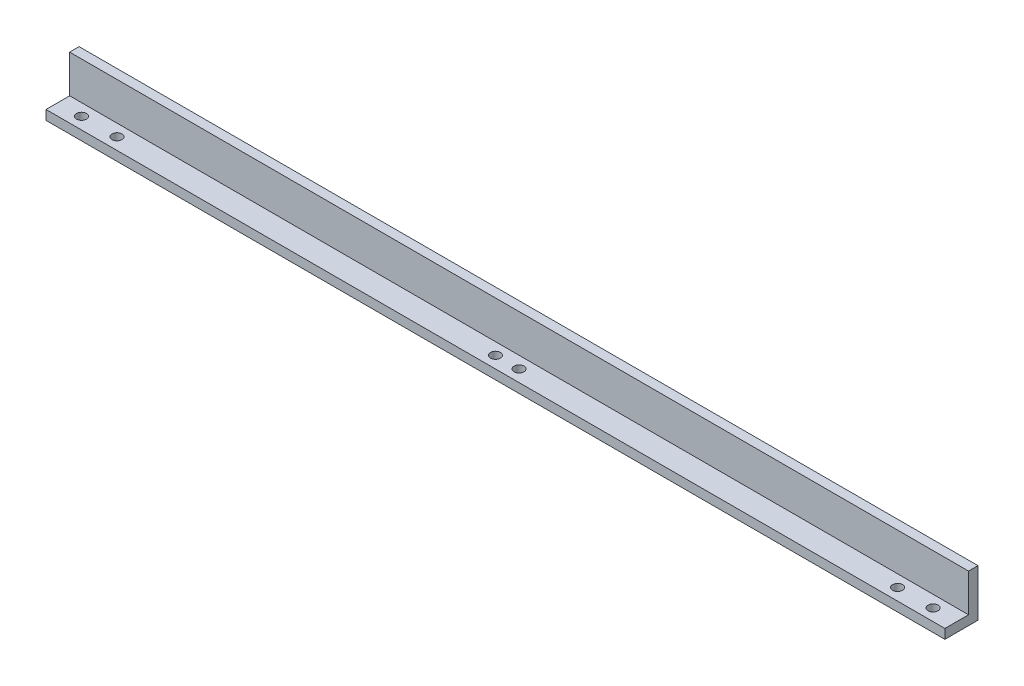
SolidWorks part; units mm, degrees
ref_plane "Front Plane" through (0, 0, 0) normal (0, 0, 1) x (1, 0, 0)
ref_plane "Top Plane" through (0, 0, 0) normal (0, 1, 0) x (1, 0, 0)
ref_plane "Right Plane" through (0, 0, 0) normal (1, 0, 0) x (0, 0, -1)
sketch "Sketch1" plane through (0, 0, 0) normal (0, 1, 0) x (1, 0, 0)
  line L0 (0, 32.2946) -> (0, -41.7959) construction
  line L1 (-190, -5) -> (190, -5)
  line L2 (-190, -5) -> (-190, 5)
  line L3 (-190, 5) -> (190, 5)
  line L4 (190, -5) -> (190, 5)
  line L5 (-190, -5) -> (190, 5) construction
  line L6 (-190, 5) -> (190, -5) construction
  circle A0 centre (-180, 0) radius 2.1
  circle A1 centre (-165, 0) radius 2.1
  circle A2 centre (165, 0) radius 2.1
  circle A3 centre (180, 0) radius 2.1
  circle A4 centre (5, 0) radius 2.1
  circle A5 centre (-5, 0) radius 2.1
  point P0 (0, 0)
  dimension "D3" = 4.2
  dimension "D4" = 4.2
  dimension "D6" = 15
  dimension "D7" = 4.2
  dimension "D8" = 4.2
  dimension "D9" = 5
  dimension "D10" = 5
  dimension "D1" = 10
  dimension "D2" = 380
  dimension "D5" = 10
extrude "Boss-Extrude1" add sketch "Sketch1" along normal blind 4
sketch "Sketch2" plane through (0, 0, -5) normal (0, 0, -1) x (-1, 0, 0)
  line L1 (-190, 0) -> (190, 0)
  line L2 (-190, 0) -> (-190, 20)
  line L3 (-190, 20) -> (190, 20)
  line L4 (190, 0) -> (190, 20)
  dimension "D1" = 380
  dimension "D2" = 20
extrude "Boss-Extrude2" add sketch "Sketch2" along normal blind 4
